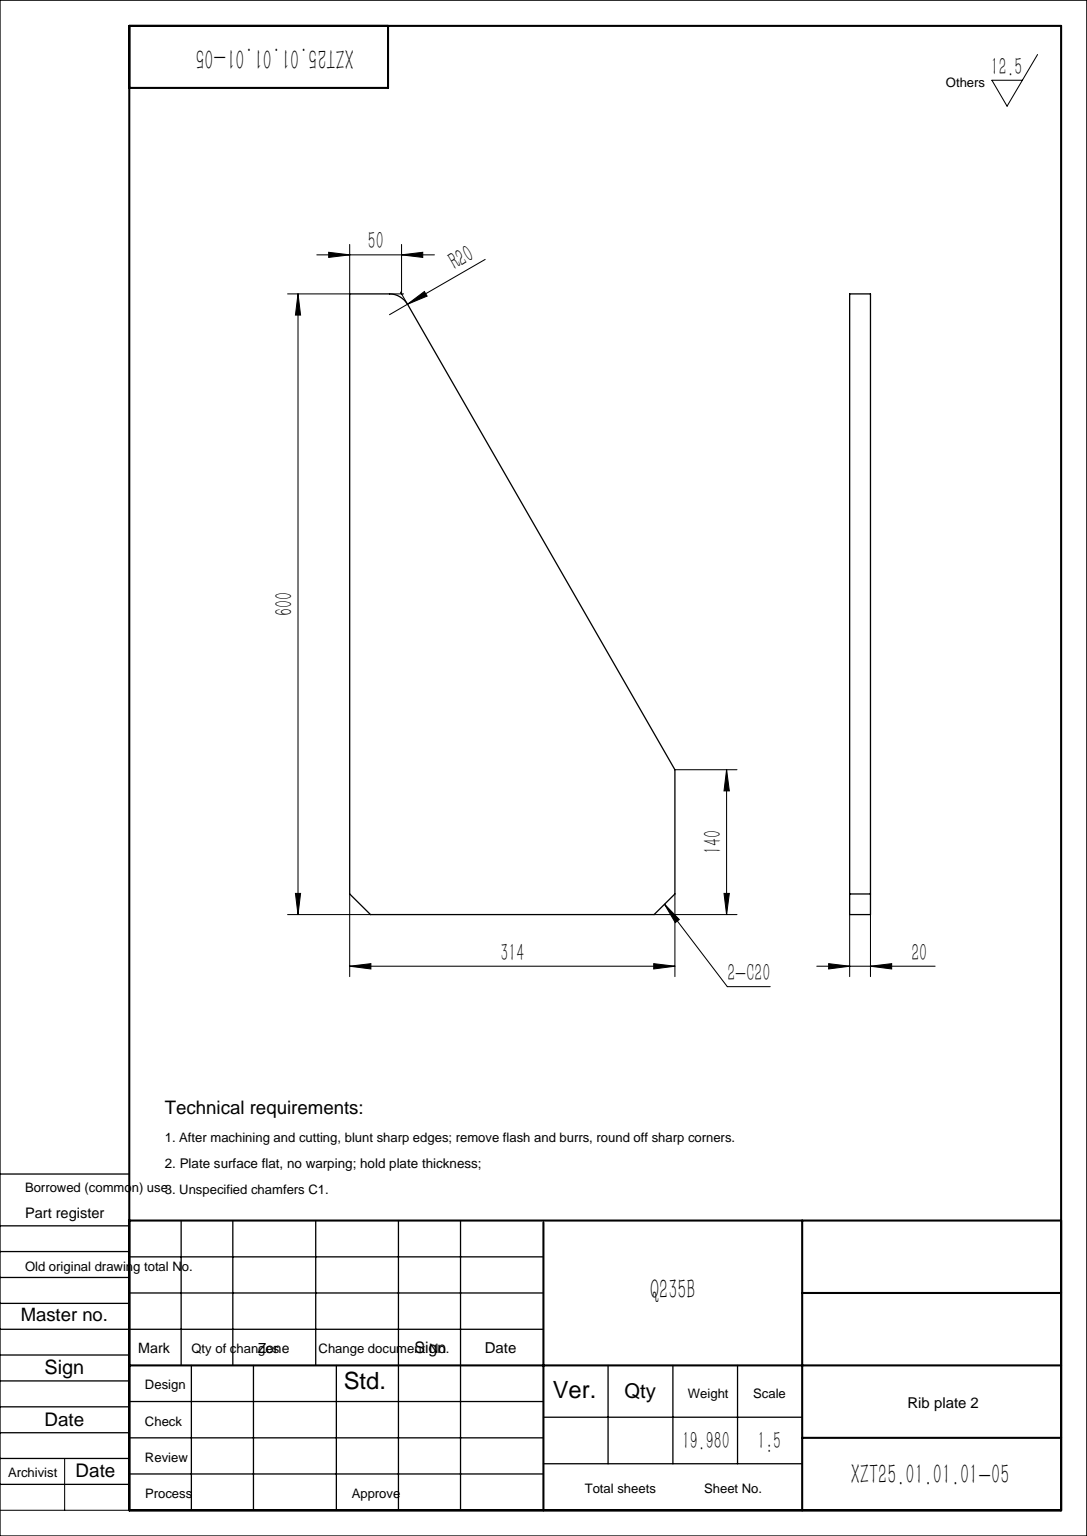
SolidWorks part; units mm, degrees
material "Q235B"
ref_plane "Front Plane" through (0, 0, 0) normal (0, 0, 1) x (1, 0, 0)
ref_plane "Top Plane" through (0, 0, 0) normal (0, 1, 0) x (1, 0, 0)
ref_plane "Right Plane" through (0, 0, 0) normal (1, 0, 0) x (0, 0, -1)
sketch "Sketch1" plane through (0, 0, 0) normal (0, 0, 1) x (1, 0, 0)
  line L0 (0, 0) -> (314, 0)
  line L1 (314, 0) -> (314, 140)
  line L2 (314, 140) -> (50, 600)
  line L3 (50, 600) -> (0, 600)
  line L4 (0, 600) -> (0, 0)
  dimension "D1" = 140
  dimension "D2" = 314
  dimension "D3" = 600
  dimension "D4" = 50
extrude "Boss-Extrude1" add sketch "Sketch1" along normal mid plane 20
fillet "Fillet1" radius 20 1 edges at (50, 600, 0)
chamfer "Chamfer1" distance 20 angle 45 2 edges at (314, 0, 0) (0, 0, 0)
